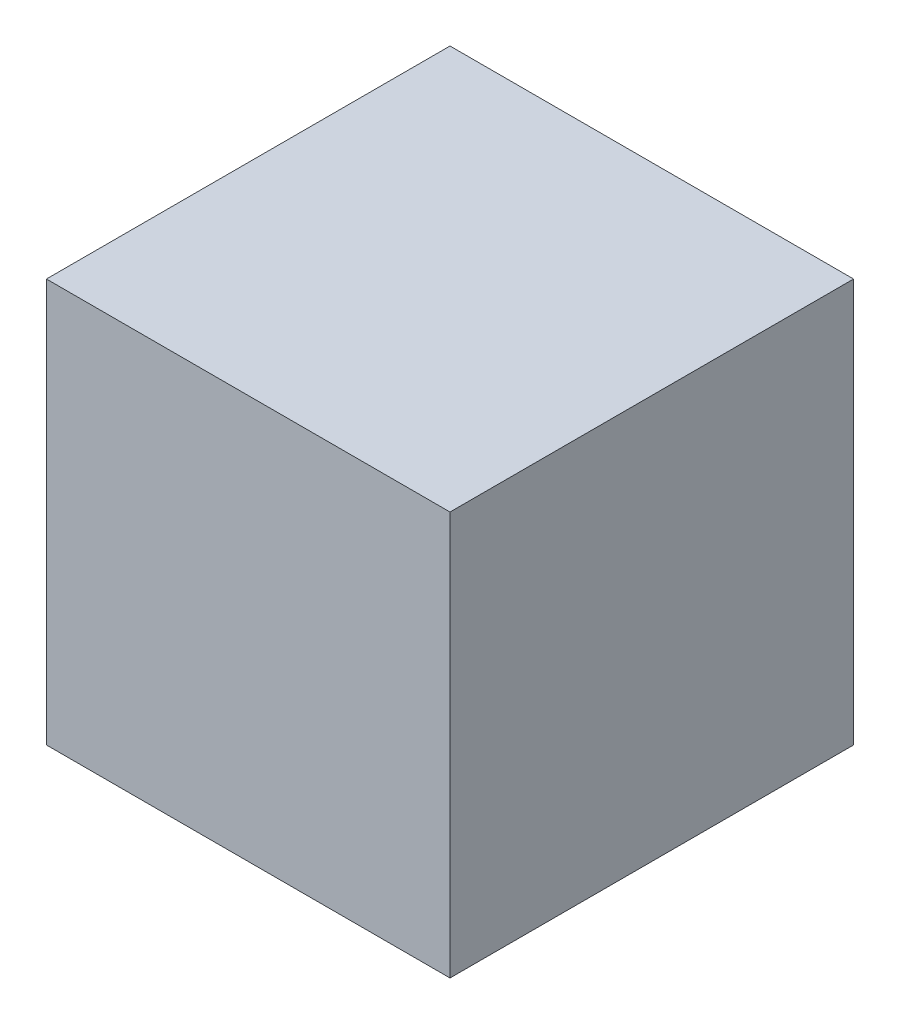
SolidWorks part; units mm, degrees
material "SS400B"
ref_plane "Front Plane" through (0, 0, 0) normal (0, 0, 1) x (1, 0, 0)
ref_plane "Top Plane" through (0, 0, 0) normal (0, 1, 0) x (1, 0, 0)
ref_plane "Right Plane" through (0, 0, 0) normal (1, 0, 0) x (0, 0, -1)
sketch "Sketch1" plane through (0, 0, 0) normal (0, 1, 0) x (1, 0, 0)
  line L1 (-12.5, 12.5) -> (12.5, 12.5)
  line L2 (-12.5, 12.5) -> (-12.5, -12.5)
  line L3 (-12.5, -12.5) -> (12.5, -12.5)
  line L4 (12.5, 12.5) -> (12.5, -12.5)
  line L5 (-12.5, 12.5) -> (12.5, -12.5) construction
  line L6 (-12.5, -12.5) -> (12.5, 12.5) construction
  point P0 (0, 0)
  dimension "D1" = 25
  dimension "D2" = 25
extrude "Boss-Extrude1" add sketch "Sketch1" along normal blind 25
